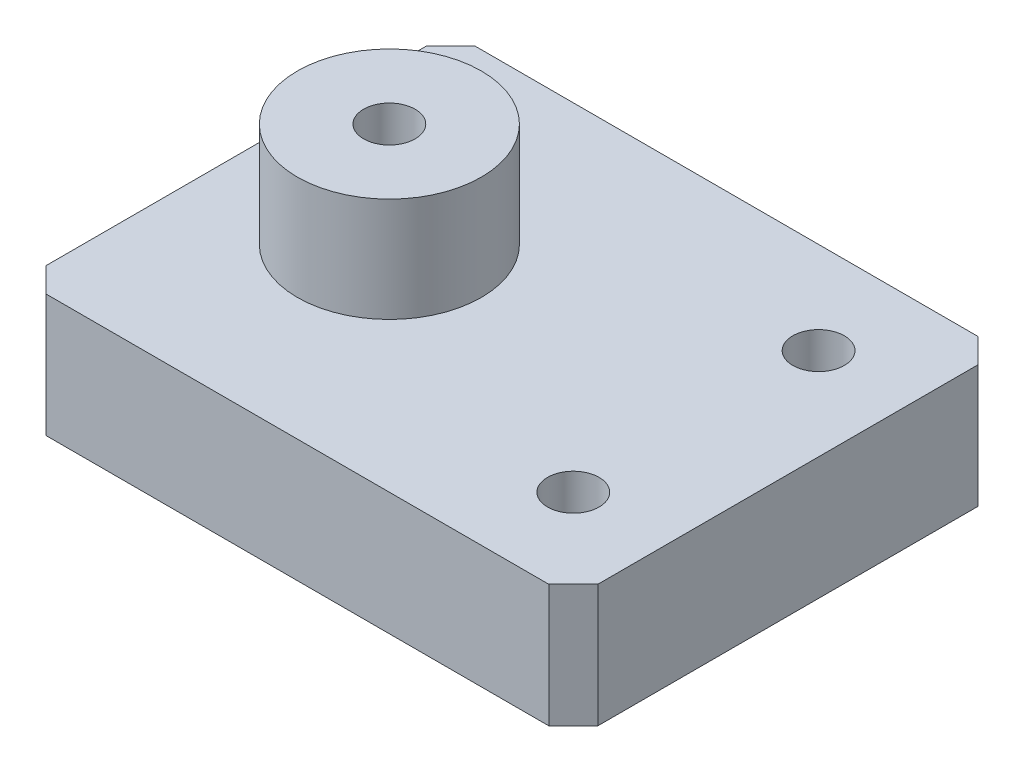
from build123d import *

# Parameters (mm, degrees)
SKETCH_1_W         = 45
SKETCH_1_H         = 35
EXTRUDE_1_DEPTH    = 5
CHAMFER_1_SIZE     = 2
SKETCH_8_R         = 7.5
EXTRUDE_2_DEPTH    = 8.5
HOLE_WIZARD_M5_1_D = 4.2
HOLE_WIZARD_M5_2_D = 4.2


with BuildPart() as part:
    # 草图1 → 凸台-拉伸1 (new, symmetric)
    with BuildSketch(Plane(origin=(0, 0, 0), x_dir=(1, 0, 0), z_dir=(0, 1, 0))):
        Rectangle(SKETCH_1_W, SKETCH_1_H)
    extrude(amount=EXTRUDE_1_DEPTH, both=True)

    # 倒角1
    chamfer_1_edges = [part.edges().sort_by_distance(p)[0] for p in [
        (22.5, 0, 17.5),
        (-22.5, 0, 17.5),
        (-22.5, 0, -17.5),
        (22.5, 0, -17.5),
    ]]
    chamfer(chamfer_1_edges, length=CHAMFER_1_SIZE)

    # 草图8 → 凸台-拉伸2 (add)
    with BuildSketch(Plane(origin=(0, 5, 0), x_dir=(1, 0, 0), z_dir=(0, 1, 0))):
        with Locations(Location((-10, 0, 0), (0, 0, 90))):
            Circle(SKETCH_8_R)
    extrude(amount=EXTRUDE_2_DEPTH)

    # M5 螺纹孔1 (through all)
    with Locations(Plane(origin=(0, 5, 0), x_dir=(1, 0, 0), z_dir=(0, 1, 0))):
        with Locations((15, -10), (15, 10)):
            Hole(HOLE_WIZARD_M5_1_D / 2)

    # M5 螺纹孔2 (through all)
    with Locations(Plane(origin=(0, 13.5, 0), x_dir=(1, 0, 0), z_dir=(0, 1, 0))):
        with Locations((-10, 0)):
            Hole(HOLE_WIZARD_M5_2_D / 2)


solid = part.part
